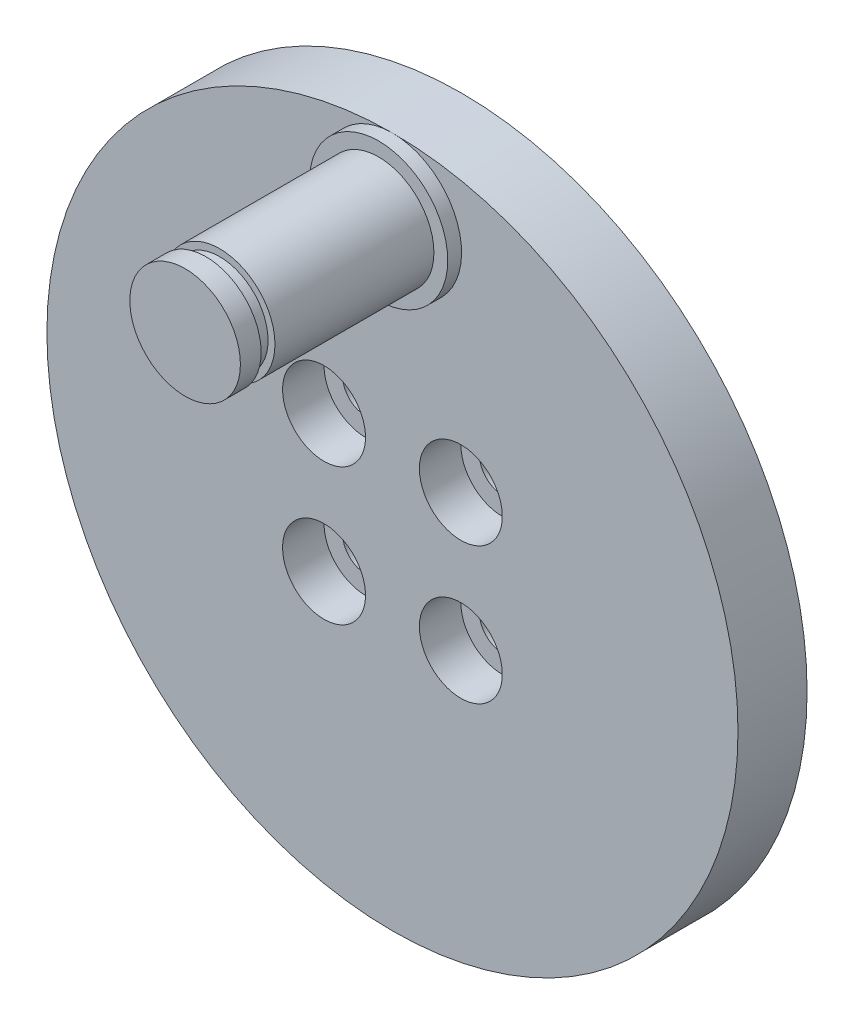
from build123d import *

# Parameters (mm, degrees)
SKETCH_1_R               = 25
EXTRUDE_1_DEPTH          = 5
SKETCH_4_R               = 4
EXTRUDE_2_DEPTH          = 15
SKETCH_6_R               = 1.65
CUT_EXTRUDE_2_DEPTH      = 10
PATTERN_CIRCULAR_1_COUNT = 4
SKETCH_7_R               = 3
CUT_EXTRUDE_3_DEPTH      = 3
SKETCH_8_R               = 5
SKETCH_8_R_2             = 4
EXTRUDE_3_DEPTH          = 1
CUT_EXTRUDE_START        = -2.5
SKETCH_10_R              = 4
SKETCH_10_R_2            = 3.5
CUT_EXTRUDE_4_DEPTH      = 1


with BuildPart() as part:
    # 草图1 → 凸台-拉伸1 (new body)
    with BuildSketch(Plane.XY):
        Circle(SKETCH_1_R)
    extrude(amount=EXTRUDE_1_DEPTH)

    # 草图4 → 凸台-拉伸2 (add)
    with BuildSketch(Plane.XY.offset(5)):
        with Locations((0, 20)):
            Circle(SKETCH_4_R)
    extrude(amount=EXTRUDE_2_DEPTH)

    # 草图6 → 切除-拉伸2 (cut)
    with BuildSketch(Plane(origin=(0, 0, 0), x_dir=(-1, 0, 0), z_dir=(0, 0, -1))):
        with Locations((4.949747468, 4.949747468)):
            Circle(SKETCH_6_R)
    cut_extrude_2 = extrude(amount=-CUT_EXTRUDE_2_DEPTH, mode=Mode.SUBTRACT)

    # 阵列(圆周)1: 切除-拉伸2 ×4 about axis
    pattern_circular_1_axis = Axis((0, 0, 0), (0, 0, 1))
    for i in range(1, PATTERN_CIRCULAR_1_COUNT):
        add(cut_extrude_2.rotate(pattern_circular_1_axis, i * 360 / PATTERN_CIRCULAR_1_COUNT), mode=Mode.SUBTRACT)

    # 草图7 → 切除-拉伸3 (cut)
    with BuildSketch(Plane(origin=(0, 0, 5), x_dir=(-1, 0, 0), z_dir=(0, 0, -1))):
        with Locations((-4.949747468, 4.949747468)):
            Circle(SKETCH_7_R)
        with Locations((4.949747468, 4.949747468)):
            Circle(SKETCH_7_R)
        with Locations((4.949747468, -4.949747468)):
            Circle(SKETCH_7_R)
        with Locations((-4.949747468, -4.949747468)):
            Circle(SKETCH_7_R)
    extrude(amount=CUT_EXTRUDE_3_DEPTH, mode=Mode.SUBTRACT)

    # 草图8 → 凸台-拉伸3 (add)
    with BuildSketch(Plane.XY.offset(5)):
        with Locations(Location((0, 20, 0), (0, 0, 90))):
            Circle(SKETCH_8_R)
        with Locations((0, 20)):
            Circle(SKETCH_8_R_2, mode=Mode.SUBTRACT)
    extrude(amount=EXTRUDE_3_DEPTH)

    # 草图10 → 切除-拉伸4 (cut)
    with BuildSketch(Plane.XY.offset(20).offset(CUT_EXTRUDE_START)):
        with Locations((0, 20)):
            Circle(SKETCH_10_R)
        with Locations((0, 20)):
            Circle(SKETCH_10_R_2, mode=Mode.SUBTRACT)
    extrude(amount=CUT_EXTRUDE_4_DEPTH, mode=Mode.SUBTRACT)


solid = part.part
